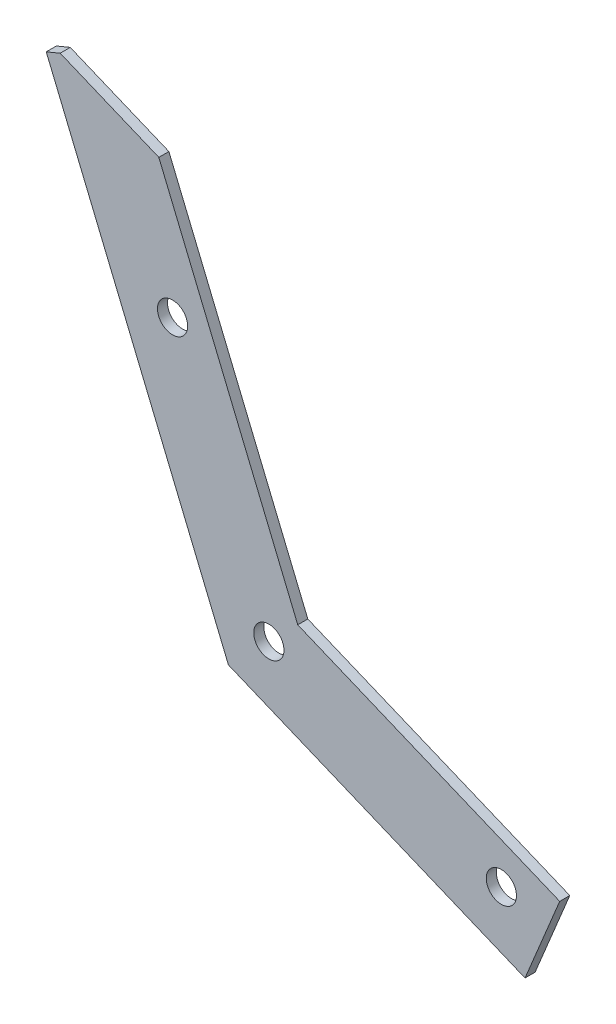
from build123d import *

# Parameters (mm, degrees)
BOSS_EXTRUDE1_DEPTH = 310
SHELL1_T            = -2
CUT_EXTRUDE1_DEPTH  = 10
CUT_EXTRUDE2_DEPTH  = 397.026111511
CUT_EXTRUDE3_DEPTH  = 5
SKETCH5_R           = 3
CUT_EXTRUDE4_DEPTH  = 10
CUT_EXTRUDE5_DEPTH  = 397.026111511
CUT_EXTRUDE7_DEPTH  = 382.100397819
CUT_EXTRUDE8_DEPTH  = 211.562851919


with BuildPart() as part:
    # Sketch1 → Boss-Extrude1 (new body)
    with BuildSketch(Plane.XY):
        Polygon((-174.265144247, 0), (-123.224065222, -123.224065222), (0, -174.265144247), (123.224065222, -123.224065222), (174.265144247, 0), (123.224065222, 123.224065222), (0, 174.265144247), (-123.224065222, 123.224065222), align=None)
    extrude(amount=BOSS_EXTRUDE1_DEPTH)

    # Shell1
    shell1_openings = [part.faces().sort_by_distance(p)[0] for p in [
        (0, 0, 0),
    ]]
    offset(amount=SHELL1_T, openings=shell1_openings, kind=Kind.INTERSECTION)

    # Sketch2 → Cut-Extrude1 (cut)
    with BuildSketch(Plane.XY.offset(310)):
        Polygon((104.089893603, 104.089893603), (0, 147.20533924), (-104.089893603, 104.089893603), (-147.20533924, 0), (-104.089893603, -104.089893603), (0, -147.20533924), (104.089893603, -104.089893603), (147.20533924, 0), align=None)
    extrude(amount=-CUT_EXTRUDE1_DEPTH, mode=Mode.SUBTRACT)

    # Sketch3 → Cut-Extrude2 (cut, through all)
    with BuildSketch(Plane.XY.offset(310)):
        Polygon((70.138181093, 169.328548035), (-63.801020235, -154.029288344), (130.028007017, -234.315900213), (263.967208344, 89.041936166), align=None)
    extrude(amount=-CUT_EXTRUDE2_DEPTH, mode=Mode.SUBTRACT)

    # Sketch4 → Cut-Extrude3 (cut)
    with BuildSketch(Plane.XY.offset(310)):
        Polygon((-143.932898959, 151.622295845), (-51.544945707, 113.353952609), (-116.60112921, -43.705567918), (-208.989082461, -5.437224682), align=None)
    extrude(amount=-CUT_EXTRUDE3_DEPTH, mode=Mode.SUBTRACT)

    # Sketch5 → Cut-Extrude4 (cut)
    with BuildSketch(Plane.XY.offset(310)):
        with Locations((0, 155.323280742)):
            Circle(SKETCH5_R)
        with Locations((-46.193976626, 136.189109124)):
            Circle(SKETCH5_R)
        with Locations((46.193976626, 136.189109124)):
            Circle(SKETCH5_R)
        with Locations((-128.964316707, -63.636168463)):
            Circle(SKETCH5_R)
        with Locations((-109.830145089, -109.830145089)):
            Circle(SKETCH5_R)
        with Locations((-63.636168463, -128.964316707)):
            Circle(SKETCH5_R)
    extrude(amount=-CUT_EXTRUDE4_DEPTH, mode=Mode.SUBTRACT)

    # Sketch19 → Cut-Extrude5 (cut, through all)
    with BuildSketch(Plane.XY.offset(310)):
        Polygon((-32.528091751, -78.529760263), (61.612032611, 148.744604734), (-87.132572124, 210.356637345), (-181.272696485, -16.917727653), align=None)
    extrude(amount=-CUT_EXTRUDE5_DEPTH, mode=Mode.SUBTRACT)

    # Sketch21 → Cut-Extrude7 (cut, through all)
    with BuildSketch(Plane.XY.offset(310)):
        Polygon((-117.866497168, -117.866497168), (-58.933248584, -142.277448007), (-61.612032611, -148.744604734), (-123.224065222, -123.224065222), (-164.354968833, -23.925279891), (-155.209028079, -27.713652592), align=None)
    extrude(amount=-CUT_EXTRUDE7_DEPTH, mode=Mode.SUBTRACT)

    # Sketch22 → Cut-Extrude8 (cut, through all)
    with BuildSketch(Plane.XY.offset(310)):
        Polygon((-154.060977781, -30.48529119), (-155.209028079, -27.713652592), (-151.289339184, -29.337240892), align=None)
    extrude(amount=-CUT_EXTRUDE8_DEPTH, mode=Mode.SUBTRACT)


solid = part.part
